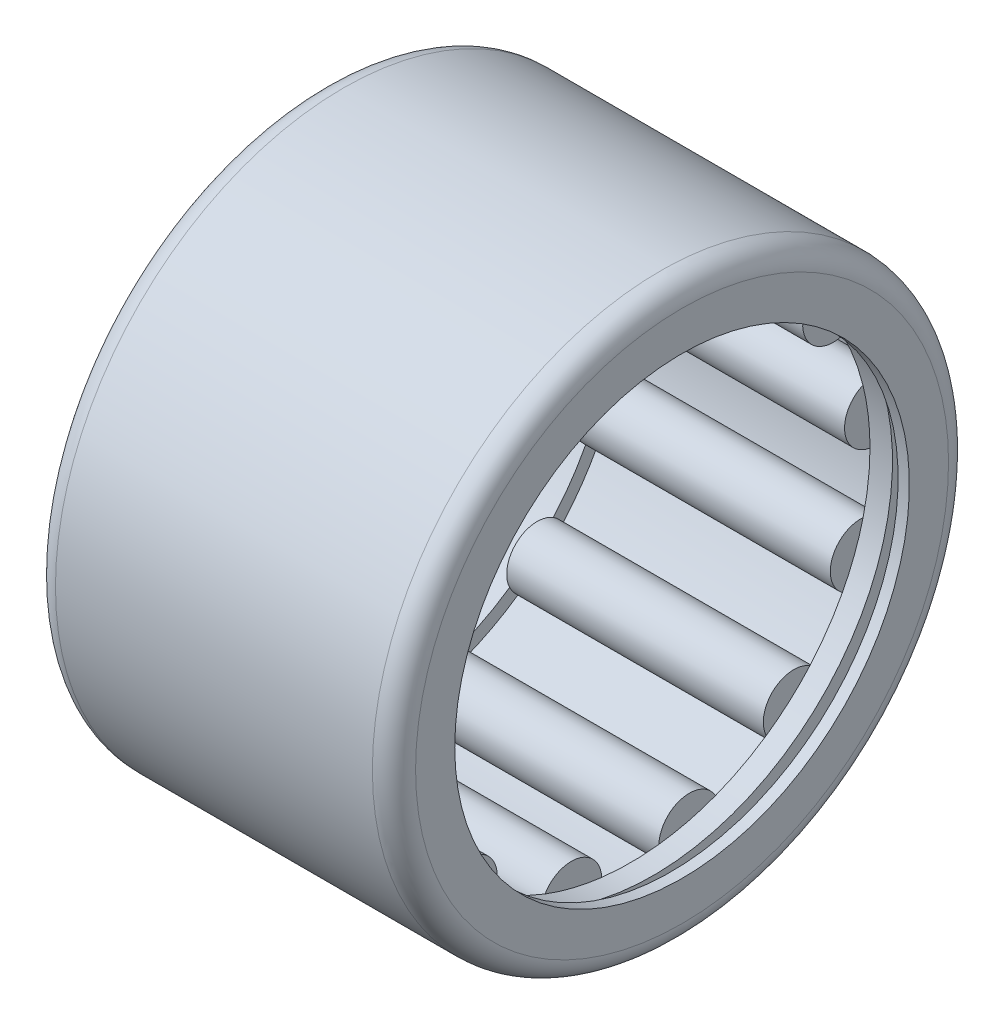
SolidWorks part; units mm, degrees
ref_plane "Front Plane" through (0, 0, 0) normal (0, 0, 1) x (1, 0, 0)
ref_plane "Top Plane" through (0, 0, 0) normal (0, 1, 0) x (1, 0, 0)
ref_plane "Right Plane" through (0, 0, 0) normal (1, 0, 0) x (0, 0, -1)
sketch "Dimension Sketch" plane through (0, 0, 0) normal (0, 0, 1) x (1, 0, 0)
  line L0 (0, 0) -> (16, 0)
  point P3 (12, 0)
  point P4 (10, 0)
  point P7 (0.6, 0)
sketch "Sketch1" plane through (0, 0, 0) normal (0, 0, 1) x (1, 0, 0)
  line L0 (0, 0) -> (3.6532, 0) construction
  line L1 (0, 0) -> (0, 6.2937) construction
  line L2 (0, 6) -> (10, 6)
  line L3 (0, 6.3125) -> (0, 8)
  line L4 (0, 8) -> (10, 8)
  line L5 (10, 6.3125) -> (10, 8)
  line L6 (0, 6.3125) -> (0.3125, 6.3125)
  line L7 (9.6875, 6.3125) -> (9.6875, 7.6875)
  line L8 (0.3125, 7.6875) -> (9.6875, 7.6875)
  line L9 (0.3125, 6.3125) -> (0.3125, 7.6875)
  line L10 (-4.6031, 6.8438) -> (23.1053, 6.8438) construction
  line L11 (9.6875, 6.3125) -> (10, 6.3125)
  line L12 (5, 8) -> (5, 6) construction
  line L13 (1.4375, 13) -> (1.4375, 10)
  line L14 (8.5625, 7.6875) -> (8.5625, 10)
  line L15 (1.4375, 13) -> (1.4375, 10)
  line L16 (8.5625, 13) -> (8.5625, 10)
  line L17 (1.125, 13) -> (1.125, 10)
  line L18 (8.875, 13) -> (8.875, 10)
  line L19 (0.8125, 13) -> (0.8125, 10)
  line L20 (9.1875, 7.6875) -> (9.1875, 6)
  line L21 (0.8125, 6.6562) -> (9.1875, 6.6562)
  line L22 (0.8125, 7.0312) -> (9.1875, 7.0312)
sketch "Sketch5" plane through (0, 0, 0) normal (0, 0, 1) x (1, 0, 0)
  line L1 (0.8125, 6.6562) -> (9.1875, 6.6562) construction
  line L2 (0.8125, 7.0312) -> (9.1875, 7.0312) construction
  line L3 (1.4375, 13) -> (1.4375, 10) construction
  line L4 (0.8125, 13) -> (0.8125, 10) construction
  line L6 (0.8125, 6.6562) -> (1.4375, 6.6562)
  line L7 (0.8125, 7.0312) -> (1.4375, 7.0312)
  line L8 (1.4375, 7.0312) -> (1.4375, 6.6562)
  line L9 (0.8125, 7.0312) -> (0.8125, 6.6562)
  line L14 (0, 0) -> (3.6532, 0) construction
  line L15 (0, 0) -> (3.6532, 0) construction
revolve "Base-Revolve2" add sketch "Sketch5" angle 360 about L15
sketch "Sketch6" plane through (0, 0, 0) normal (0, 0, 1) x (1, 0, 0)
  line L0 (-4.6031, 6.8438) -> (23.1053, 6.8438) construction
  line L4 (0.8125, 6.6562) -> (9.1875, 6.6562) construction
  line L5 (1.4375, 13) -> (1.4375, 10) construction
  line L6 (-4.6031, 6.8438) -> (23.1053, 6.8438) construction
  line L7 (1.125, 13) -> (1.125, 10) construction
  line L8 (1.125, 6.6562) -> (1.4375, 6.6562) construction
  line L9 (1.4375, 6.8438) -> (1.4375, 6.6562) construction
  line L10 (1.125, 6.8438) -> (1.125, 6.6562) construction
  line L11 (1.075, 6.8438) -> (1.075, 6.6063)
  line L12 (1.075, 6.6063) -> (1.4875, 6.6063)
  line L13 (1.4875, 6.8438) -> (1.4875, 6.6063)
  line L14 (1.075, 6.8438) -> (1.4875, 6.8438)
  dimension "D1" = 0.05
revolve "Cut-Revolve1" cut sketch "Sketch6" angle 360 about L6
pattern_circular "CirPattern3" count 13 over 360 about axis through (0, 0, 0) along (1, 0, 0) of "Cut-Revolve1"
sketch "Sketch3" plane through (0, 0, 0) normal (0, 0, 1) x (1, 0, 0)
  line L1 (0.3125, 7.6875) -> (9.6875, 7.6875) construction
  line L2 (8.5625, 7.6875) -> (8.5625, 10) construction
  line L3 (1.4375, 13) -> (1.4375, 10) construction
  line L4 (0.8125, 7.0312) -> (9.1875, 7.0312) construction
  line L6 (-4.6031, 6.8438) -> (23.1053, 6.8438) construction
  line L7 (1.4375, 7.6885) -> (8.5625, 7.6885)
  line L8 (2, 7.6875) -> (8.5625, 7.6875) construction
  line L9 (8.5625, 7.6885) -> (8.5625, 7.0312)
  line L10 (1.4375, 7.6885) -> (1.4375, 7.0312)
  line L11 (1.125, 7.0312) -> (1.4375, 7.0312)
  line L12 (8.875, 13) -> (8.875, 10) construction
  line L13 (-4.6031, 6.8438) -> (23.1053, 6.8438) construction
  line L14 (8.5625, 7.0312) -> (8.875, 7.0312)
  line L16 (1.125, 13) -> (1.125, 10) construction
  line L17 (8.875, 7.0312) -> (8.875, 6.8438)
  line L18 (1.125, 7.0312) -> (1.125, 6.8438)
  line L19 (1.125, 6.8438) -> (8.875, 6.8438)
  dimension "D1" = 0.001
revolve "Base-Revolve" add sketch "Sketch3" angle 360 about L13
sketch "Sketch2" plane through (0, 0, 0) normal (0, 0, 1) x (1, 0, 0)
  line L0 (0, 0) -> (3.6532, 0) construction
  line L1 (9.6875, 6.3125) -> (10, 6.3125) construction
  line L2 (0, 6.3125) -> (0.3125, 6.3125) construction
  line L3 (9.6875, 6.3125) -> (9.6875, 7.6875) construction
  line L4 (10, 6.3125) -> (10, 8) construction
  line L5 (0.3125, 7.6875) -> (9.6875, 7.6875) construction
  line L6 (0.3125, 6.3125) -> (0.3125, 7.6875) construction
  line L7 (0, 6.3125) -> (0, 8) construction
  line L8 (0, 8) -> (10, 8) construction
  line L9 (0, 0) -> (3.6532, 0) construction
  line L10 (9.6875, 6.3125) -> (10, 6.3125)
  line L11 (0, 6.3125) -> (0.3125, 6.3125)
  line L12 (9.6875, 6.3125) -> (9.6875, 7.6875)
  line L13 (10, 6.3125) -> (10, 8)
  line L14 (0.3125, 7.6875) -> (9.6875, 7.6875)
  line L15 (0.3125, 6.3125) -> (0.3125, 7.6875)
  line L16 (0, 6.3125) -> (0, 8)
  line L17 (0, 8) -> (10, 8)
revolve "Boss-Revolve2" add sketch "Sketch2" angle 360 about L9
ref_plane "Plane1" through (5, 0, 0) normal (-1, 0, 0) x (0, 0, 1)
mirror "Mirror1" about plane through (5, 0, 0) normal (-1, 0, 0) of "Base-Revolve2"
pattern_circular "CirPattern2" count 13 over 360 about axis through (0, 0, 0) along (1, 0, 0) of "Base-Revolve"
fillet "Fillet1" radius 0.6 2 edges at (0, 0, 8) (10, 0, 8)
mirror "Mirror2" about plane through (5, 0, 0) normal (-1, 0, 0) of "Base-Revolve"
equation "\"D3@Sketch1\" = \"D@Dimension Sketch\""
equation "\"D1@Sketch1\" = \"Fw@Dimension Sketch\""
equation "\"D2@Sketch1\" = \"C@Dimension Sketch\""
equation "\"D1@Fillet1\" = \"r@Dimension Sketch\""
equation "\"D4@Sketch1\" = \"D2@Sketch1\" / 32"
equation "\"D12@Sketch1\" =  ( \"D2@Sketch1\" - \"D4@Sketch1\" * 2 ) / 2 - 0.5 "
equation "\"D11@Sketch1\" = \"D12@Sketch1\""
equation "\"D8@Sketch1\" = \"D12@Sketch1\" - \"D4@Sketch1\" * 2"
equation "\"D7@Sketch1\" = \"D8@Sketch1\""
equation "\"D9@Sketch1\" = \"D4@Sketch1\"*1.2"
equation "\"D6@Sketch1\" = (  \"D8@Sketch1\" + \"D12@Sketch1\" )  / 2"
equation "\"D5@Sketch1\" = \"D6@Sketch1\""
equation "\"D1@CirPattern2\" = 3.14* ( \"D3@Sketch1\" / 2 - \"D4@Sketch1\" - \"D1@Sketch1\" / 2 )  * 2 /  ( \"D3@Sketch1\" - \"D1@Sketch1\" ) *5"
equation "\"D1@CirPattern3\" = \"D1@CirPattern2\""
